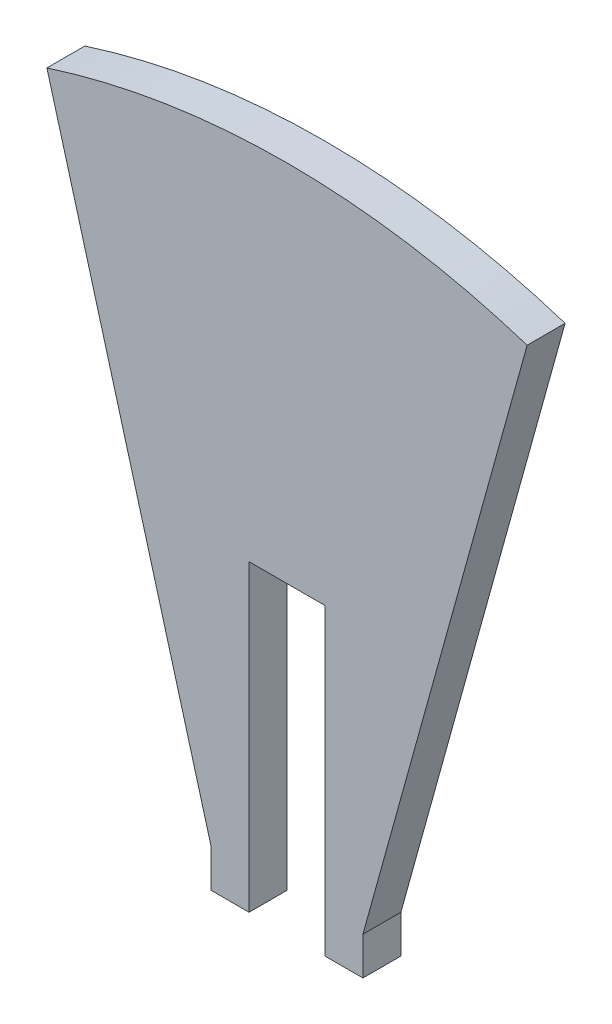
from build123d import *

# Parameters (mm, degrees)
BOSS_EXTRUDE1_DEPTH = 5
SKETCH2_W           = 20
SKETCH2_H           = 160
CUT_EXTRUDE1_DEPTH  = 10


with BuildPart() as part:
    # Sketch1 → Boss-Extrude1 (new, symmetric)
    with BuildSketch(Plane.XY):
        with BuildLine():
            Line((-63.274211694, 196.041766301), (-20, 40))
            Line((-20, 40), (-20, 30))
            Line((-20, 30), (20, 30))
            Line((20, 30), (20, 40))
            Line((20, 40), (63.274211694, 196.041766301))
            ThreePointArc((63.274211694, 196.041766301), (0, 206), (-63.274211694, 196.041766301))
        make_face()
    extrude(amount=BOSS_EXTRUDE1_DEPTH, both=True)

    # Sketch2 → Cut-Extrude1 (cut)
    with BuildSketch(Plane.XY.offset(5)):
        with Locations((0, 30)):
            Rectangle(SKETCH2_W, SKETCH2_H)
    extrude(amount=-CUT_EXTRUDE1_DEPTH, mode=Mode.SUBTRACT)


solid = part.part
